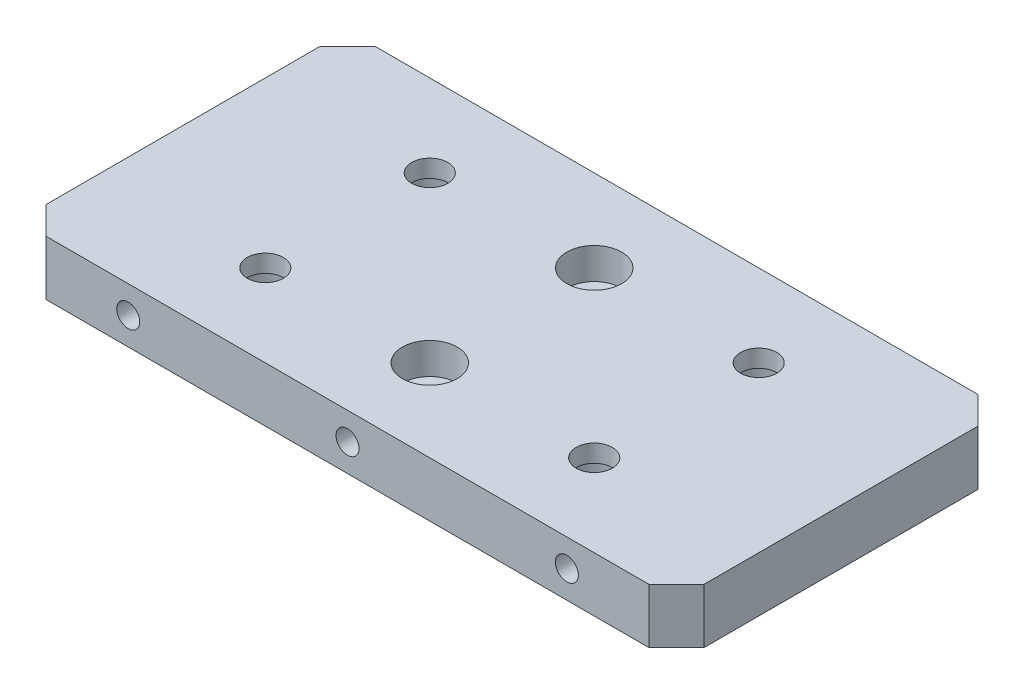
SolidWorks part; units mm, degrees
material "A6061 T6"
ref_plane "前视基准面" through (0, 0, 0) normal (0, 0, 1) x (1, 0, 0)
ref_plane "上视基准面" through (0, 0, 0) normal (0, 1, 0) x (1, 0, 0)
ref_plane "右视基准面" through (0, 0, 0) normal (1, 0, 0) x (0, 0, -1)
sketch "草图1" plane through (0, 0, 0) normal (0, 1, 0) x (1, 0, 0)
  line L1 (-60, 30) -> (60, 30)
  line L2 (-60, 30) -> (-60, -30)
  line L3 (-60, -30) -> (60, -30)
  line L4 (60, 30) -> (60, -30)
  line L5 (-60, 30) -> (60, -30) construction
  line L6 (-60, -30) -> (60, 30) construction
  point P0 (0, 0)
  dimension "D1" = 60
  dimension "D2" = 120
extrude "凸台-拉伸1" add sketch "草图1" along normal blind 10
chamfer "倒角1" distance 5 angle 45 4 edges at (-60, 5, -30) (60, 5, -30) (60, 5, 30) (-60, 5, 30)
hole_wizard "M5 螺纹孔1" positions "草图2" profile "草图3" tap size "M5" standard "GB"
sketch "草图2" plane through (0, 0, 30) normal (0, 0, 1) x (1, 0, 0)
  line L0 (-55, 10) -> (55, 10) construction
  line L1 (-60, 0) -> (-60, 10) construction
  line L2 (60, 10) -> (60, 0) construction
  point P0 (-40, 5)
  point P2 (0, 5)
  point P4 (40, 5)
  dimension "D1" = 5
  dimension "D2" = 20
  dimension "D3" = 20
  dimension "D4" = 40
sketch "草图3" plane through (-40, 5, 30) normal (1, 0, 0) x (0, -1, 0)
  line L0 (0, 0) -> (0, 13.6618)
  line L1 (0, 13.6618) -> (2.1, 12.4)
  line L2 (2.1, 12.4) -> (2.1, 0)
  line L5 (2.1, 0) -> (0, 0)
  line L10 (0, 13.6618) -> (-2.1, 12.4) construction
  line L11 (0, -6.35) -> (0, 107.95) construction
  dimension "螺纹孔钻头直径" = 4.2
  dimension "螺纹孔钻头深度" = 12.4
  dimension "导头角度" = 118
cosmetic thread "孔螺蚊线1" parameters "D1"=10, "D2"=5
cosmetic thread "孔螺蚊线2" parameters "D1"=10, "D2"=5
cosmetic thread "孔螺蚊线3" parameters "D1"=10, "D2"=5
hole_wizard "打孔尺寸(%根据)内六角圆柱头螺钉的类型1" positions "草图4" profile "草图5" counterbore size "M6" standard "GB"
sketch "草图4" plane through (0, 0, 0) normal (0, -1, 0) x (-1, 0, 0)
  line L0 (55, -30) -> (-55, -30) construction
  line L1 (-55, 30) -> (55, 30) construction
  line L2 (60, 25) -> (60, -25) construction
  line L3 (-60, -25) -> (-60, 25) construction
  point P0 (30, -15)
  point P2 (30, 15)
  point P4 (-30, -15)
  point P6 (-30, 15)
  dimension "D1" = 15
  dimension "D2" = 15
  dimension "D3" = 30
  dimension "D4" = 30
sketch "草图5" plane through (-30, 0, 15) normal (1, 0, 0) x (0, 0, -1)
  line L0 (0, 0) -> (0, 14.3828)
  line L1 (0, 14.3828) -> (3.3, 12.4)
  line L2 (3.3, 12.4) -> (3.3, 6.8)
  line L3 (3.3, 6.8) -> (5.5, 6.8)
  line L4 (5.5, 6.8) -> (5.5, 0)
  line L5 (5.5, 0) -> (0, 0)
  line L10 (0, 14.3828) -> (-3.3, 12.4) construction
  line L11 (0, -6.35) -> (0, 107.95) construction
  dimension "孔直径" = 6.6
  dimension "孔深度" = 12.4
  dimension "柱形沉头孔直径" = 11
  dimension "柱形沉头孔深度" = 6.8
  dimension "导头角度" = 118
hole_wizard "打孔尺寸(%根据)内六角圆柱头螺钉的类型2" positions "草图6" profile "草图7" counterbore size "M5" standard "GB"
sketch "草图6" plane through (0, 10, 0) normal (0, 1, 0) x (1, 0, 0)
  point P0 (0, -15)
  point P3 (0, 15)
sketch "草图7" plane through (0, 10, 15) normal (1, 0, 0) x (0, 0, 1)
  line L0 (0, 0) -> (0, 14.0524)
  line L1 (0, 14.0524) -> (2.75, 12.4)
  line L2 (2.75, 12.4) -> (2.75, 5.7)
  line L3 (2.75, 5.7) -> (5, 5.7)
  line L4 (5, 5.7) -> (5, 0)
  line L5 (5, 0) -> (0, 0)
  line L10 (0, 14.0524) -> (-2.75, 12.4) construction
  line L11 (0, -6.35) -> (0, 107.95) construction
  dimension "孔直径" = 5.5
  dimension "孔深度" = 12.4
  dimension "柱形沉头孔直径" = 10
  dimension "柱形沉头孔深度" = 5.7
  dimension "导头角度" = 118
